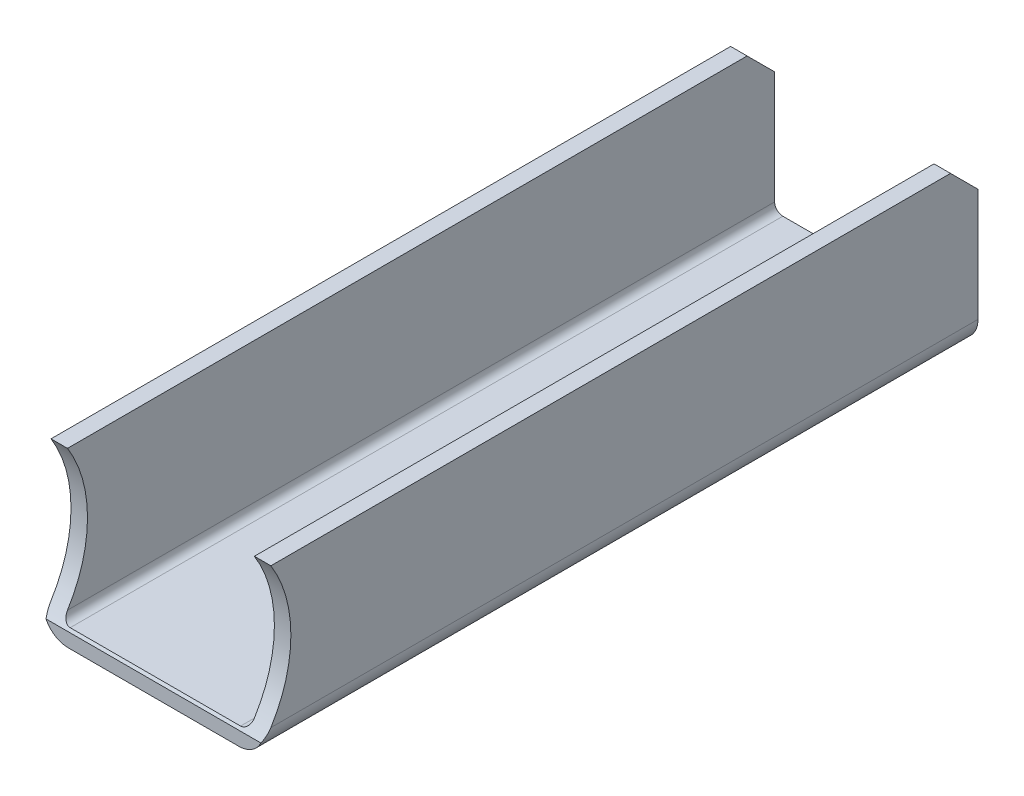
from build123d import *

# Parameters (mm, degrees)
BOSS_EXTRUDE1_DEPTH = 130
CHAMFER1_SIZE       = 5
SKETCH2_R           = 24.15
CUT_EXTRUDE1_DEPTH  = 130
CUT_EXTRUDE2_DEPTH  = 130


with BuildPart() as part:
    # Sketch1 → Boss-Extrude1 (new body)
    with BuildSketch(Plane.XY):
        with BuildLine():
            Line((0, 0), (0, -25.5))
            ThreePointArc((0, -25.5), (1.318019485, -28.681980515), (4.5, -30))
            Line((4.5, -30), (35.5, -30))
            ThreePointArc((35.5, -30), (38.681980515, -28.681980515), (40, -25.5))
            Line((40, -25.5), (40, 0))
            Line((40, 0), (37, 0))
            Line((37, 0), (37, -25.5))
            ThreePointArc((37, -25.5), (36.560660172, -26.560660172), (35.5, -27))
            Line((35.5, -27), (4.5, -27))
            ThreePointArc((4.5, -27), (3.439339828, -26.560660172), (3, -25.5))
            Line((3, -25.5), (3, 0))
            Line((3, 0), (0, 0))
        make_face()
    extrude(amount=BOSS_EXTRUDE1_DEPTH)

    # Chamfer1
    chamfer1_edges = [part.edges().sort_by_distance(p)[0] for p in [
        (38.5, 0, 0),
        (1.5, 0, 0),
    ]]
    chamfer(chamfer1_edges, length=CHAMFER1_SIZE)

    # Sketch2 → Cut-Extrude1 (cut)
    with BuildSketch(Plane(origin=(40, 0, 0), x_dir=(0, 0, -1), z_dir=(1, 0, 0))):
        with Locations((-149.15, -12.75)):
            Circle(SKETCH2_R)
    extrude(amount=-CUT_EXTRUDE1_DEPTH, mode=Mode.SUBTRACT)

    # Sketch3 → Cut-Extrude2 (cut)
    with BuildSketch(Plane.XZ.offset(30)):
        with BuildLine():
            Line((24.5, 96), (24.5, 21))
            ThreePointArc((24.5, 21), (20, 16.5), (15.5, 21))
            Line((15.5, 21), (15.5, 96))
            ThreePointArc((15.5, 96), (20, 100.5), (24.5, 96))
        make_face()
    extrude(amount=-CUT_EXTRUDE2_DEPTH, mode=Mode.SUBTRACT)


solid = part.part
